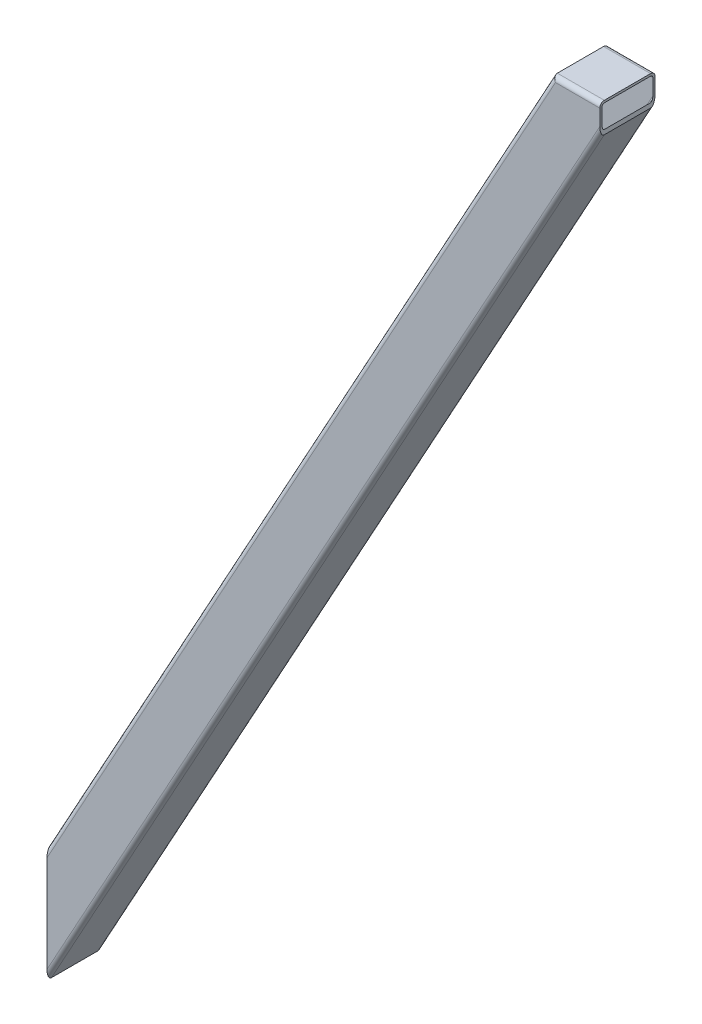
SolidWorks part; units mm, degrees
material "1023 碳钢板 (SS)"
ref_plane "Front Plane" through (0, 0, 0) normal (0, 0, 1) x (1, 0, 0)
ref_plane "Top Plane" through (0, 0, 0) normal (0, 1, 0) x (1, 0, 0)
ref_plane "Right Plane" through (0, 0, 0) normal (1, 0, 0) x (0, 0, -1)
sketch "Sketch1" plane through (0, 0, 0) normal (0, 0, 1) x (1, 0, 0)
  line L0 (0, 0) -> (0, 208.7368)
  line L1 (0, 208.7368) -> (915, 1874.4333)
  line L2 (915, 1874.4333) -> (1000, 1874.4333)
  line L3 (1000, 1874.4333) -> (1000, 1820.4333)
  line L4 (1000, 1820.4333) -> (0, 0)
  dimension "D1" = 85
  dimension "D2" = 2124.5
  dimension "54" = 54
  dimension "D3" = 1000
extrude "Boss-Extrude1" add sketch "Sketch1" along normal blind 100 contours L4 L0 L1 L2 L3
shell "Shell1" thickness 4
fillet "Fillet1" radius 8.2 6 edges at (500, 910.2167, 0) (457.5, 1041.5851, 0) (957.5, 1874.4333, 0) (957.5, 1874.4333, 100) (500, 910.2167, 100) (457.5, 1041.5851, 100)
fillet "Fillet2" radius 4.2 6 edges at (958.6832, 1870.4333, 96) (958.6832, 1870.4333, 4) (500, 918.5247, 96) (500, 918.5247, 4) (458.6832, 1035.431, 4) (458.6832, 1035.431, 96)
sketch "Sketch2" plane through (0, 0, 0) normal (0, 0, -1) x (-1, 0, 0)
  line L1 (0, 17.0315) -> (0, 191.7053) construction
  circle A0 centre (-316, 708.43) radius 9.9785
  dimension "D1" = 708.43
  dimension "D2" = 316
hole_wizard "M8 Tapped Hole1" positions "Sketch3" profile "Sketch4" tap size "M8" standard "ISO"
sketch "Sketch3" plane through (0, 0, 0) normal (0, 0, -1) x (-1, 0, 0)
  point P0 (-316, 708.43)
sketch "Sketch4" plane through (316, 708.43, 0) normal (1, 0, 0) x (0, 1, 0)
  line L0 (0, 0) -> (0, 21.7929)
  line L1 (0, 21.7929) -> (3.4, 19.75)
  line L2 (3.4, 19.75) -> (3.4, 0)
  line L5 (3.4, 0) -> (0, 0)
  line L10 (0, 21.7929) -> (-3.4, 19.75) construction
  line L11 (0, -6.35) -> (0, 107.95) construction
  dimension "螺纹孔钻头直径" = 6.8
  dimension "螺纹孔钻头深度" = 19.75
  dimension "导头角度" = 118
cosmetic thread "Hole Thread Line 1" parameters "D1"=16, "D2"=8
